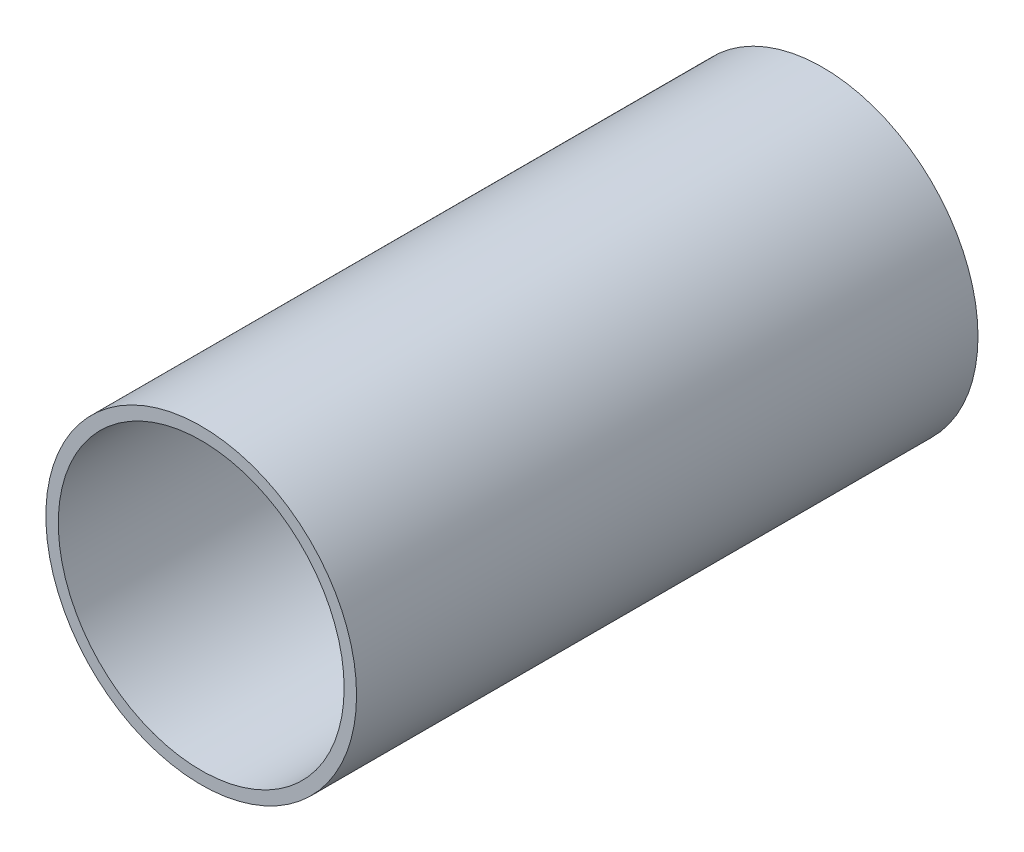
from build123d import *

# Parameters (mm, degrees)
SKETCH1_R           = 25
SKETCH1_R_2         = 23
BOSS_EXTRUDE1_DEPTH = 100


with BuildPart() as part:
    # Sketch1 → Boss-Extrude1 (new body)
    with BuildSketch(Plane.XY):
        Circle(SKETCH1_R)
        Circle(SKETCH1_R_2, mode=Mode.SUBTRACT)
    extrude(amount=BOSS_EXTRUDE1_DEPTH)


solid = part.part
